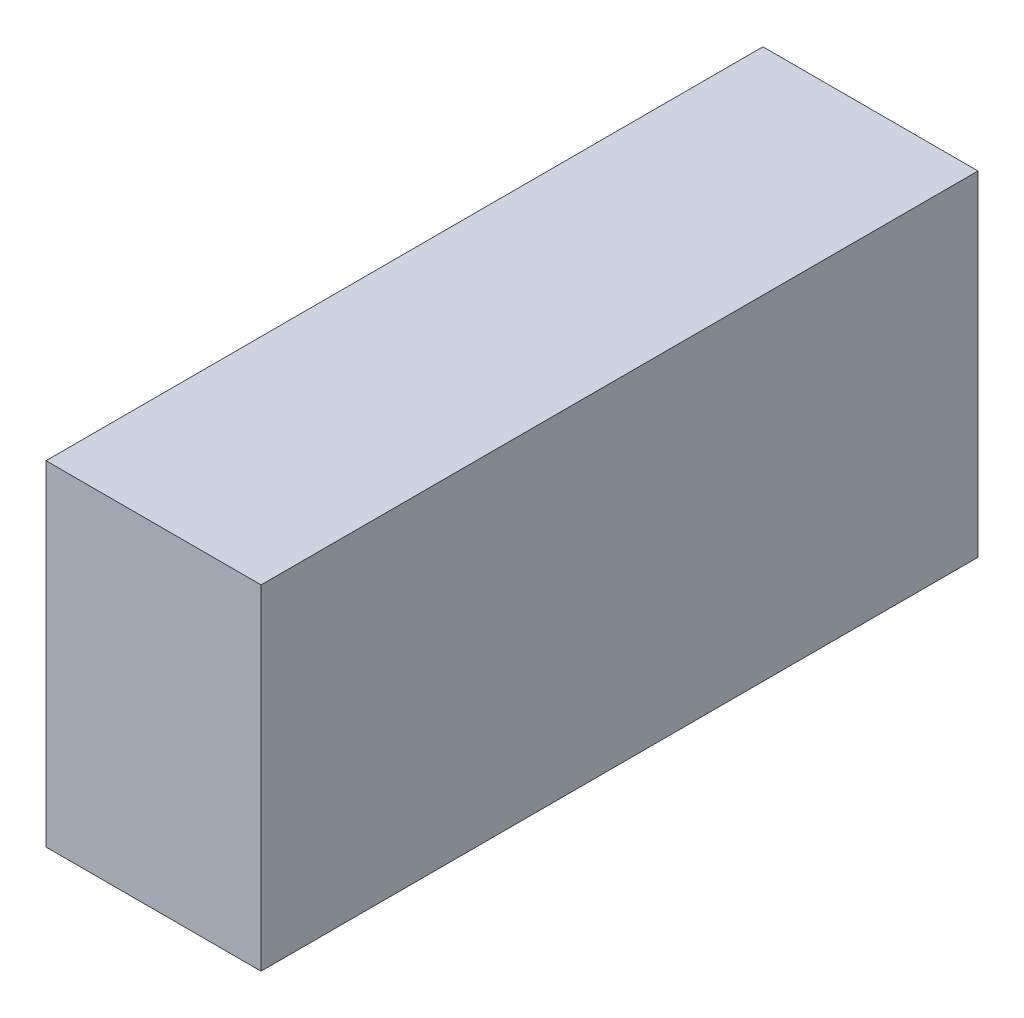
SolidWorks part; units mm, degrees
ref_plane "Front Plane" through (0, 0, 0) normal (0, 0, 1) x (1, 0, 0)
ref_plane "Top Plane" through (0, 0, 0) normal (0, 1, 0) x (1, 0, 0)
ref_plane "Right Plane" through (0, 0, 0) normal (1, 0, 0) x (0, 0, -1)
sketch "Sketch1" plane through (0, 0, 0) normal (0, 1, 0) x (1, 0, 0)
  line L3 (-4.5, 15) -> (4.5, 15)
  line L4 (-4.5, 15) -> (-4.5, -15)
  line L5 (-4.5, -15) -> (4.5, -15)
  line L6 (4.5, 15) -> (4.5, -15)
  line L7 (-4.5, 15) -> (4.5, -15) construction
  line L8 (-4.5, -15) -> (4.5, 15) construction
  point P0 (0, 0)
  dimension "D1" = 30
  dimension "D2" = 9
extrude "Boss-Extrude1" add sketch "Sketch1" along normal blind 14
